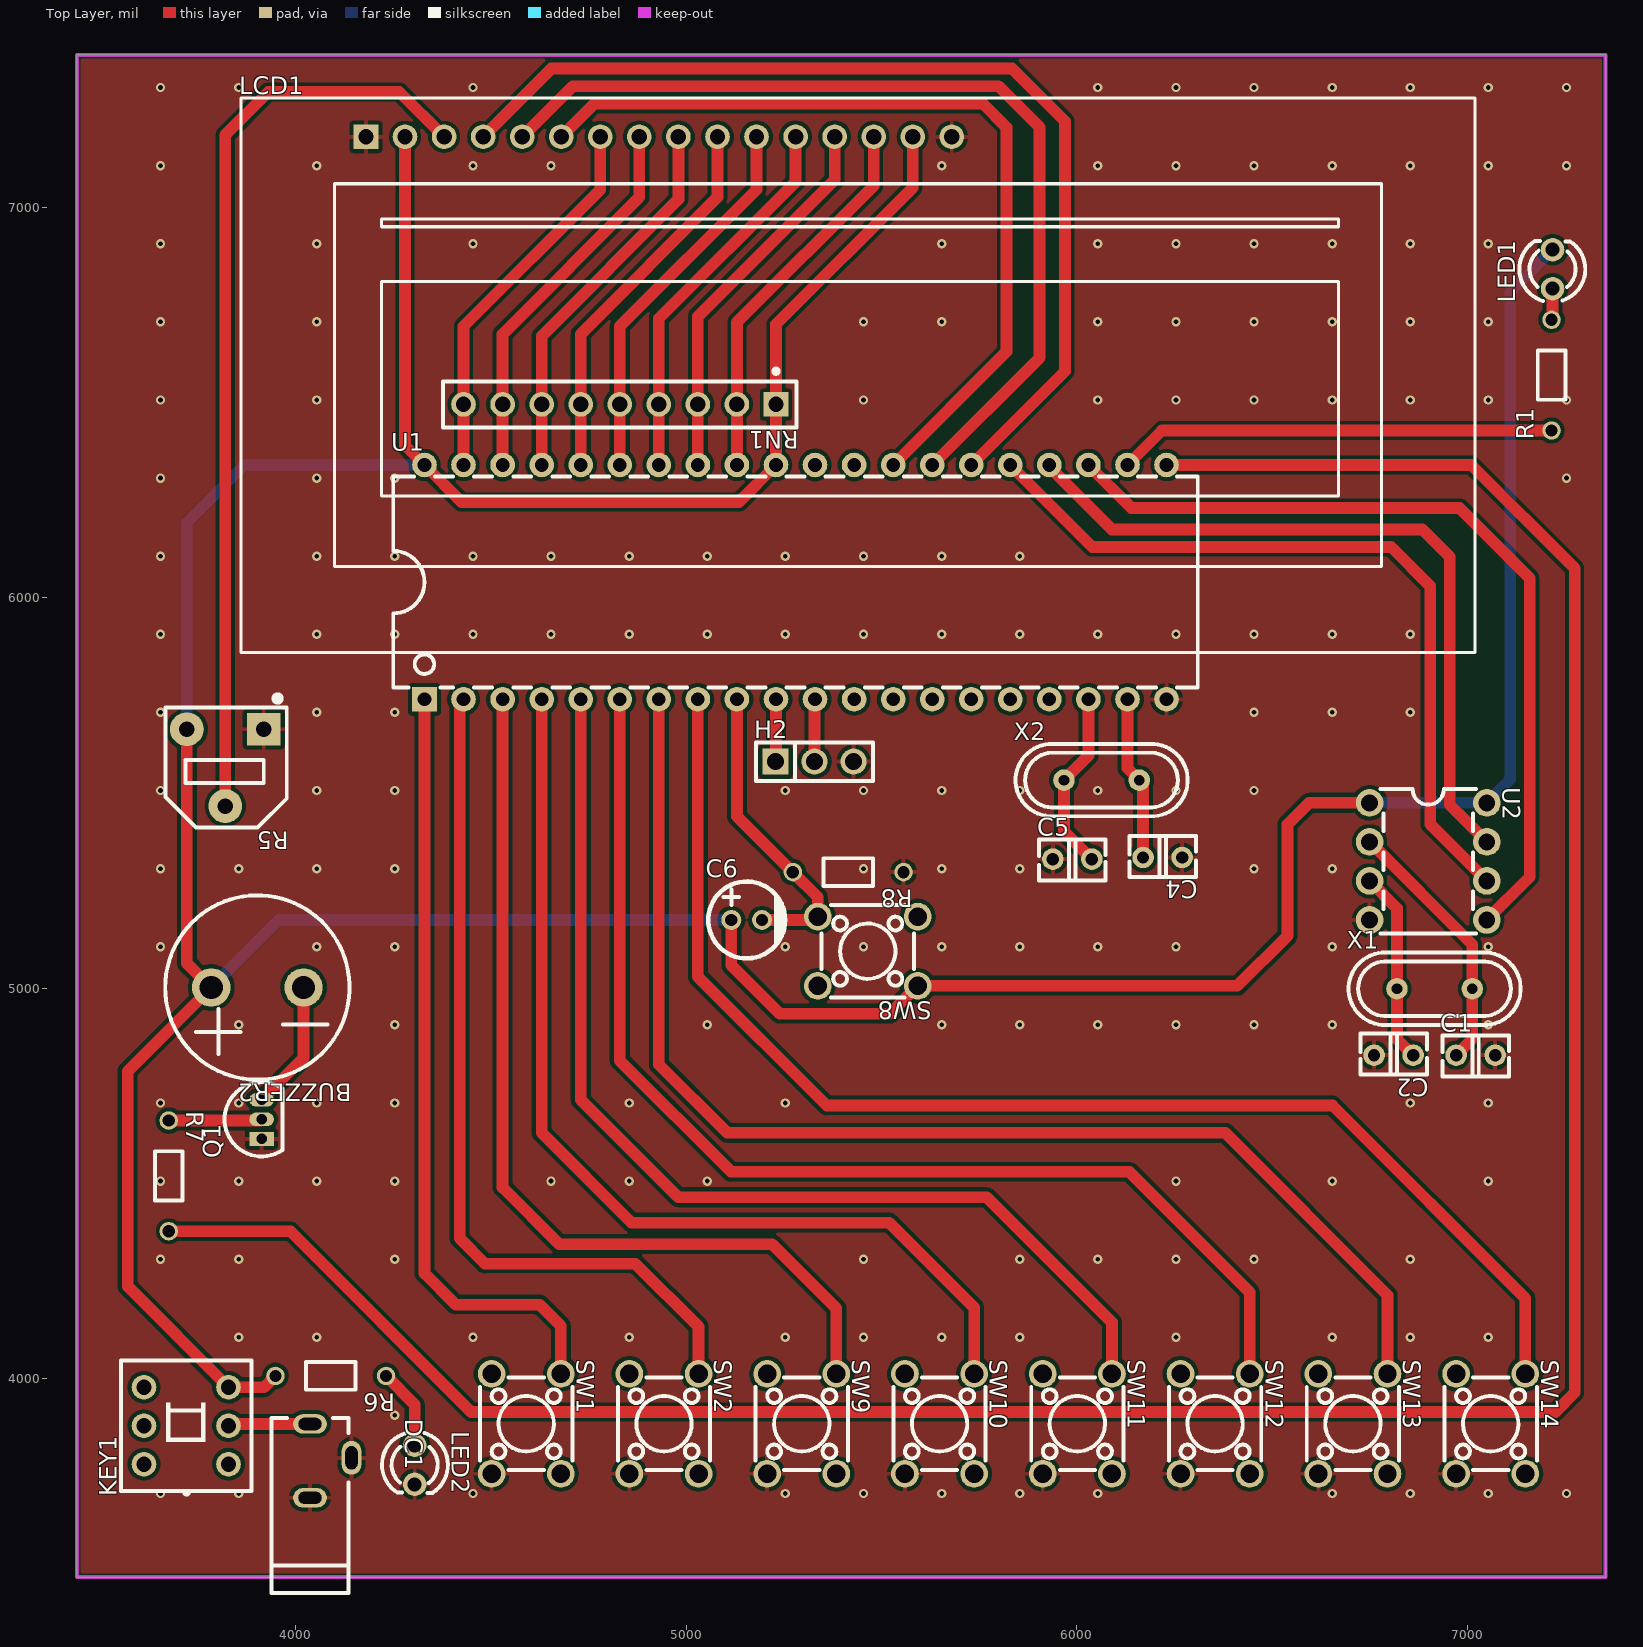
[diagram p0: Top Layer view]
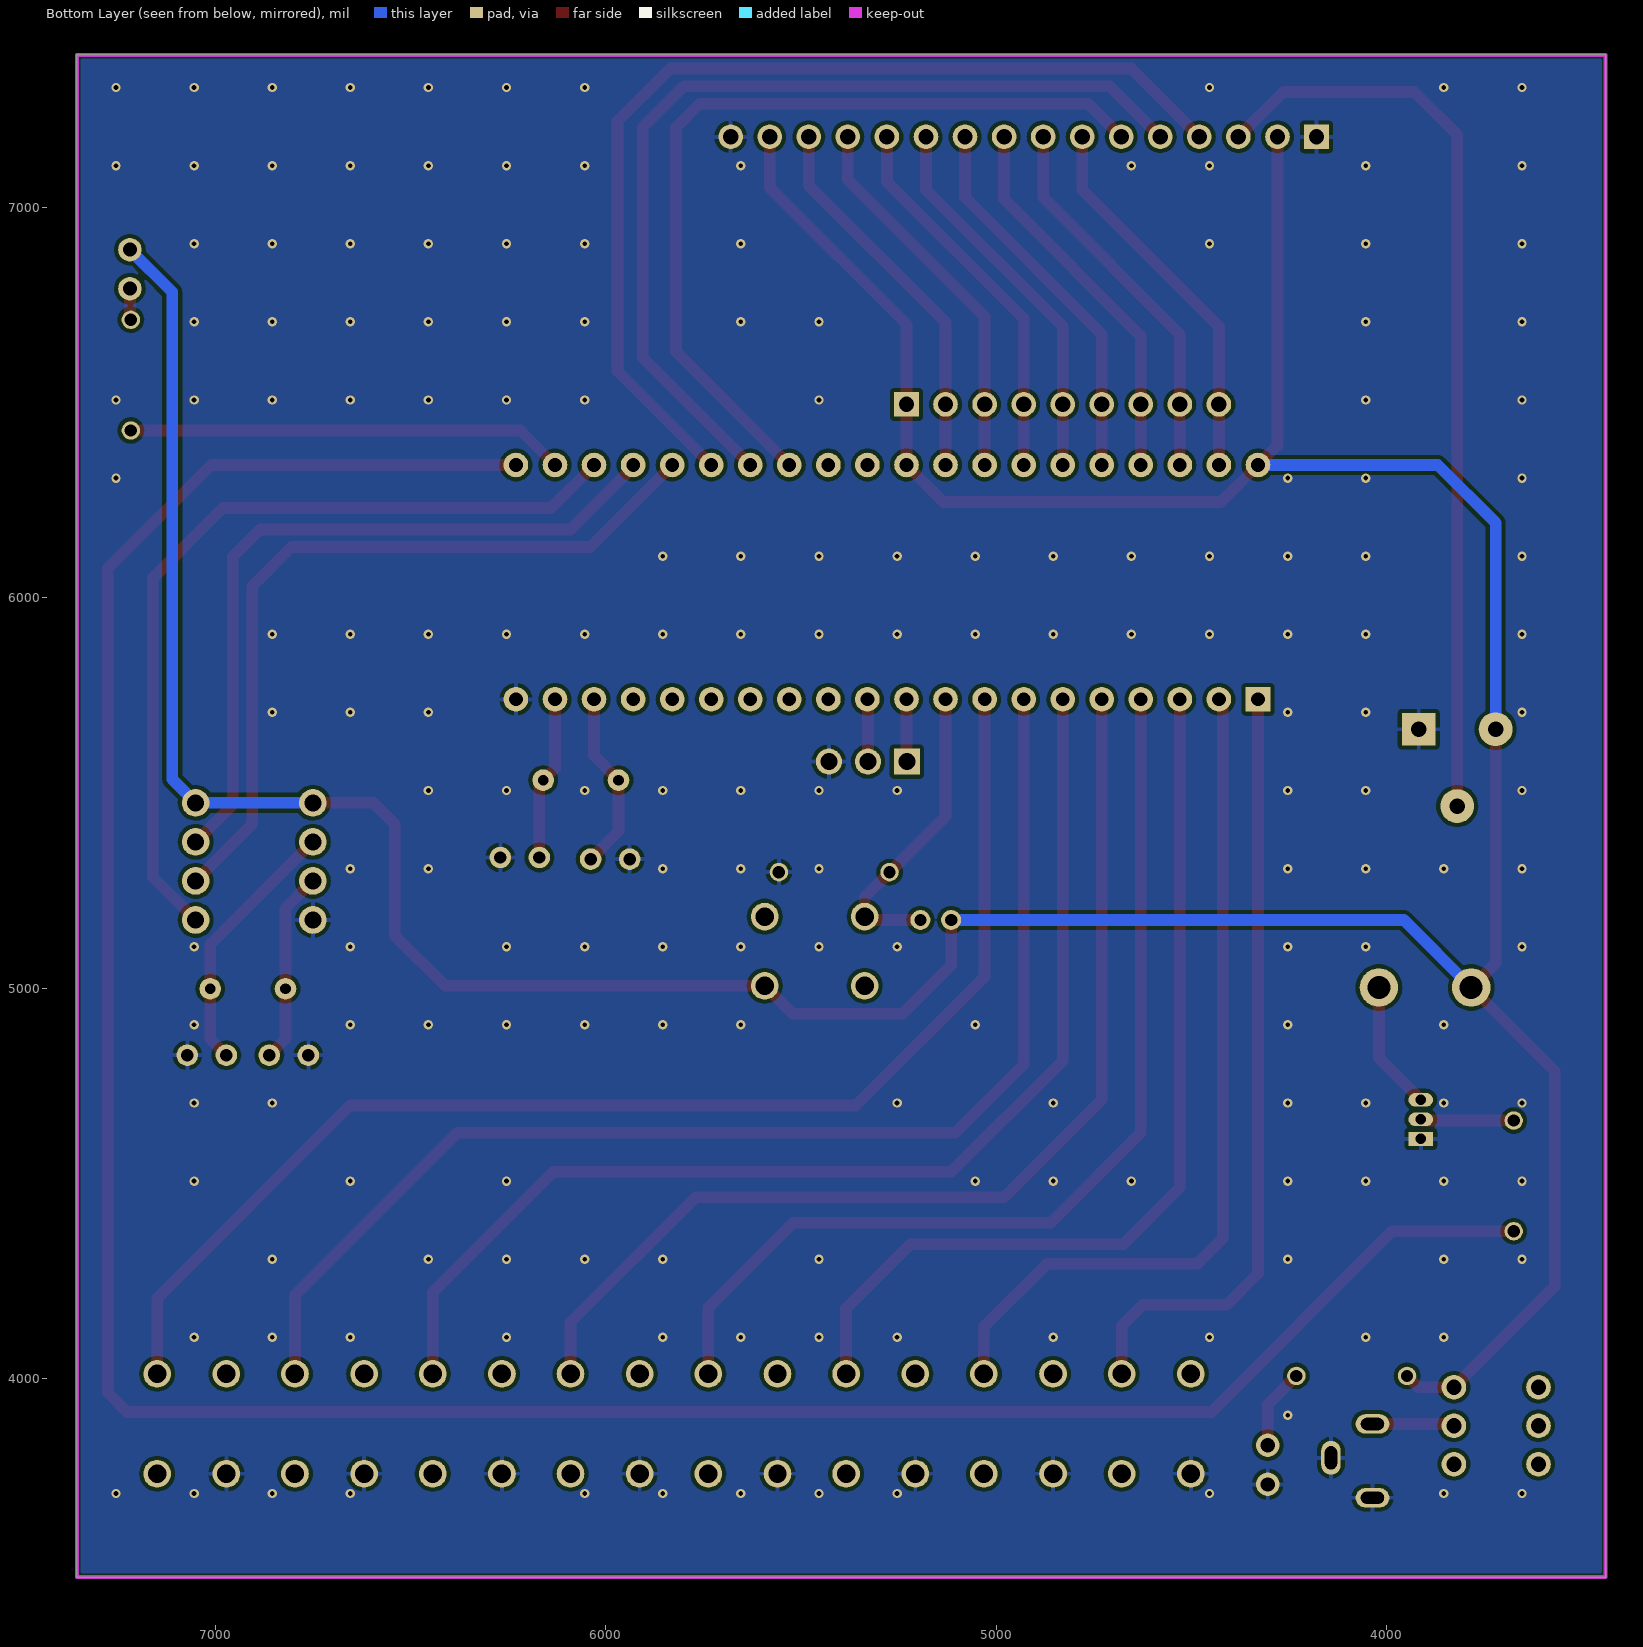
[diagram p1: Bottom Layer view, seen from below]
# Altium PCB MISC51000.pcbdoc
Units mil, origin at the board's own origin, x right, y up, seen from the top; angles counter-clockwise.
Board outline 3914.17 x 3897.64 mil, 2 copper layers (Top Layer, Bottom Layer), stack 62.206 mil thick; 32 components, 45 nets, 155 pads, 181 vias.

## Layer stack, top to bottom
Top Solder Mask Layer: solder mask 0.394, Dk 3.3
Top Layer: signal copper 1.379
Dielectric1: surface 59.449, FR4, Dk 4.5
Bottom Layer: signal copper 1.378
Bottom Solder Mask Layer: solder mask 0.394, Dk 3.3

## Board outline
3440,7390 3440,3492.36 7354.17,3492.36 7354.17,7390

## Design rules (kind name [scope] priority, off if disabled: settings)
BoardOutlineClearance copperThickness2oz_1 [All] p2 off: genericclearance=7.99 ignorepadtopadclearanceinfootprint=FALSE except(0: Arc-SplitContinuation Track-SplitContinuation SMDPad-SplitContinuation THPad-SplitContinuation Via-SplitContinuation Fill-SplitContinuation Region-SplitContinuation Poly-SplitContinuation Text-SplitContinuation Hole-SplitContinuation; 5.98: Arc-CutoutEdge SMDPad-CutoutEdge THPad-CutoutEdge Via-CutoutEdge Fill-CutoutEdge Region-CutoutEdge Text-CutoutEdge; 6.93: Hole-OutlineEdge Hole-CutoutEdge; 10: Poly-OutlineEdge Poly-CutoutEdge; 11.81: Arc-OutlineEdge Track-OutlineEdge SMDPad-OutlineEdge THPad-OutlineEdge Via-OutlineEdge Fill-OutlineEdge Region-OutlineEdge Text-OutlineEdge Track-CutoutEdge)
BoardOutlineClearance copperThickness1oz_1 [All] p4: genericclearance=4.02 ignorepadtopadclearanceinfootprint=FALSE except(0: Arc-SplitContinuation Track-SplitContinuation SMDPad-SplitContinuation THPad-SplitContinuation Via-SplitContinuation Fill-SplitContinuation Region-SplitContinuation Poly-SplitContinuation Text-SplitContinuation Hole-SplitContinuation; 6: SMDPad-CutoutEdge THPad-CutoutEdge Via-CutoutEdge Fill-CutoutEdge Region-CutoutEdge Text-CutoutEdge; 6.93: Hole-OutlineEdge Hole-CutoutEdge; 10: Poly-OutlineEdge Poly-CutoutEdge; 11.8: Arc-OutlineEdge Track-OutlineEdge SMDPad-OutlineEdge THPad-OutlineEdge Via-OutlineEdge Fill-OutlineEdge Region-OutlineEdge Text-OutlineEdge; 11.81: Arc-CutoutEdge Track-CutoutEdge)
Clearance copperThickness2oz [All] p1 off: gap=7.99 ignorepadtopadclearanceinfootprint=FALSE except(5.98: SMDPad-Track SMDPad-SMDPad THPad-Track SMDPad-THPad THPad-THPad Track-Via SMDPad-Via THPad-Via Via-Via Fill-Track Region-Track Fill-SMDPad Region-SMDPad Fill-THPad Region-THPad Fill-Via Region-Via Fill-Fill Fill-Region Region-Region Arc-Track Arc-SMDPad Arc-THPad Arc-Via Fill-Arc Region-Arc Arc-Arc Text-Track SMDPad-Text Text-THPad Text-Via Fill-Text Region-Text Arc-Text Text-Text; 6.93: Hole-Track Hole-SMDPad Hole-THPad Hole-Via Fill-Hole Region-Hole Hole-Arc Hole-Text; 10: Poly-Track Poly-SMDPad Poly-THPad Poly-Via Poly-Fill Poly-Region Poly-Poly Poly-Arc Poly-Text Poly-Hole)
Clearance copperThickness1oz [All] p3: gap=4.02 ignorepadtopadclearanceinfootprint=FALSE except(5.98: SMDPad-Track SMDPad-SMDPad THPad-Track SMDPad-THPad THPad-THPad Track-Via SMDPad-Via THPad-Via Via-Via Fill-Track Region-Track Fill-SMDPad Region-SMDPad Fill-THPad Region-THPad Fill-Via Region-Via Fill-Fill Fill-Region Region-Region; 6: Arc-Track Arc-SMDPad Arc-THPad Arc-Via Fill-Arc Region-Arc Arc-Arc Text-Track SMDPad-Text Text-THPad Text-Via Fill-Text Region-Text Arc-Text Text-Text; 6.93: Hole-Track Hole-SMDPad Hole-THPad Hole-Via Fill-Hole Region-Hole Hole-Arc Hole-Text; 10: Poly-Track Poly-SMDPad Poly-THPad Poly-Via Poly-Fill Poly-Region Poly-Poly Poly-Arc Poly-Text Poly-Hole)
Creepage creepage [All] p1: checkdistance=0 ignoreinternallayers=TRUE applytopolygonpour=TRUE
DiffPairsRouting differentialPair [All] p1: maxlimit=6 minlimit=6 mostfreqgap=6 toplayer_minwidth=5 toplayer_prefwidth=10 toplayer_maxwidth=100 toplayer_mingap=6 toplayer_prefgap=6 toplayer_maxgap=6 bottomlayer_minwidth=5 bottomlayer_prefwidth=10 bottomlayer_maxwidth=100 bottomlayer_mingap=6 bottomlayer_prefgap=6 bottomlayer_maxgap=6 maxuncoupledlength=10
HoleToHoleClearance otherClearance [All] p1: gap=11.81 allowstackedmicrovias=TRUE
Length netLength [All] p1: minlimit=0 maxlimit=0
MatchedLengths netLengthTolerance [All] p1: tolerance=1000
PasteMaskExpansion pasteMaskExpansion [All] p1: expansion=0
PlaneConnect innerPlane [All] p1: planeconnectstyle=Relief reliefexpansion=20 reliefentries=4 reliefconductorwidth=10 reliefairgap=10
PolygonConnect copperRegion [(InNet('GND'))] p1: connectstyle=Relief reliefconductorwidth=10 reliefentries=4 polygonreliefangle="90 Angle" airgapwidth=10 via.connectstyle=Relief via.reliefconductorwidth=10 via.reliefentries=4 via.polygonreliefangle="90 Angle" via.airgapwidth=10
RoutingVias viaSize [All] p1: holewidth=12.01 width=24.02 viastyle="Through Hole" minholewidth=11.81 minwidth=19.68 maxholewidth=248.03 maxwidth=393.7
SolderMaskExpansion solderMaskExpansion [IsVia] p1: expansion=-1000 istentingtop=TRUE
SolderMaskExpansion solderMaskExpansion [All] p2: expansion=2 istentingtop=FALSE
Width copperThickness2oz_2 [All] p1 off: maxlimit=100 minlimit=8 preferedwidth=10
Width copperThickness1oz_2 [All] p2: maxlimit=100 minlimit=5 preferedwidth=10

## Components (designator, comment, footprint, x,y, rotation, side; value= is the part's Value field where it differs from the comment)
BUZZER2 "buzzer" BUZ-TH_BD12.0-P6.00-D0.9-RD 3902.2,5002.04 r180 top
C1 "1nF" CAP-TH_L3.8-W2.5-P2.54-D0.50 7021.44,4828.83 r0 top
C2 "1nF" CAP-TH_L3.8-W2.5-P2.54-D0.50 6811.44,4828.83 r180 top
C4 "22pF" CAP-TH_L3.8-W2.5-P2.54-D0.50 6220,5335 r180 top
C5 "22pF" CAP-TH_L3.8-W2.5-P2.54-D0.50 5988.8,5330.73 r0 top
C6 "10uF" CAP-TH_BD5.0-P2.00-D0.8-FD-10UF50VC110GL 5155,5175 r0 top
DC1 "DC-002" DC-IN-TH_DC-3510 4090,3790 r270 top
H2 "" HDR-TH_3P-P2.54-V-M 5328.8,5580.46 r0 top
KEY1 "Non-latching switch 8.5×8.5 silent" SW-TH_6P-L8.5-W8.5-P2.54 3720,3880 r90 top
LCD1 "HS1602A" LCD1602 5440,6570 r0 top
LED1 "" LED_TH-3mm 7218.4,6841.27 r90 top
LED2 "" LED_TH-3mm 4305,3780 r270 top
Q1 "" S8050_TO_92 3913.08,4664.57 r90 top
R1 "100" Res_1/8W 7218.4,6570.02 r90 top
R5 "10kΩ" RES-ADJ-SMD_RM065-V1 3820,5565 r180 top
R6 "1kΩ" Res_1/8W 4090,4010 r180 top
R7 "10kΩ" Res_1/8W 3672.75,4519.71 r270 top
R8 "10kΩ" Res_1/8W 5415,5300 r180 top
RN1 "-" RES-ARRAY-TH_9P-P2.54-D1.0 4830,6495 r180 top
SW1 "" SW-TH_4P-L6.0-W6.0-P4.50-LS6.5 4590.5,3885 r270 top
SW2 "" SW-TH_4P-L6.0-W6.0-P4.50-LS6.5 4943.28,3885 r270 top
SW8 "" SW-TH_4P-L6.0-W6.0-P4.50-LS6.5 5465,5095 r180 top
SW9 "" SW-TH_4P-L6.0-W6.0-P4.50-LS6.5 5296.07,3885 r270 top
SW10 "" SW-TH_4P-L6.0-W6.0-P4.50-LS6.5 5648.85,3885 r270 top
SW11 "" SW-TH_4P-L6.0-W6.0-P4.50-LS6.5 6001.64,3885 r270 top
SW12 "" SW-TH_4P-L6.0-W6.0-P4.50-LS6.5 6354.43,3885 r270 top
SW13 "" SW-TH_4P-L6.0-W6.0-P4.50-LS6.5 6707.21,3885 r270 top
SW14 "" SW-TH_4P-L6.0-W6.0-P4.50-LS6.5 7060,3885 r270 top
U1 "STC89C52RC-40I-PDIP40" DIP-40_L52.0-W13.7-P2.54-LS15.2-BL 5280,6040 r0 top
U2 "DS1302N(XBLW)" PDIP-8_L9.3-W6.4-P2.54-LS7.6-BL 6900,5325 r270 top
X1 "11.0592MHz" OSC-TH_L11.1-W4.7-P4.88 6916.44,4998.83 r0 top
X2 "11.0592MHz" OSC-TH_L11.1-W4.7-P4.88 6063.8,5533.02 r0 top

## Footprints (in the part's own frame and the unit in brackets; to place one, negate y for a bottom-side part, rotate by r counter-clockwise, add the part's x,y. Pads: shape width x height; smd on the part's side, far side on the other; paste and mask are expansions set on the pad)
BUZ-TH_BD12.0-P6.00-D0.9-RD [mm]
  round 2.5 hole 1.5 paste+0 mask+0.05: 1(-3,0) 2(3,0)
  silkscreen extent -5.99,-5.99 5.99,5.99
CAP-TH_BD5.0-P2.00-D0.8-FD-10UF50VC110GL [mm]
  round 1.3 hole 0.8: 1(-1,0) 2(1,0)
  silkscreen extent -2.5,-2.5 2.5,2.5
CAP-TH_L3.8-W2.5-P2.54-D0.50 [mm]
  round 1.4 hole 0.8 paste+0 mask+0.05: 1(-1.27,0) 2(1.27,0)
  silkscreen extent -2.16,-1.4 2.16,1.27
DC-IN-TH_DC-3510 [mm]
  oval 1.27x2.2 hole 0.8 slot 1.5 at 90 deg: 1(-2.4,-1.35) 2(2.4,-1.35)
  oval 2.2x1.27 hole 0.8 slot 1.5 at 0 deg: 3(-0.2,1.35)
  silkscreen extent -2.8,-3.85 8.6,1.15
DIP-40_L52.0-W13.7-P2.54-LS15.2-BL [mil]
  rect 63x63 hole 35: 1(-950,-300)
  round 63 hole 35: 2(-850,-300) 3(-750,-300) 4(-650,-300) 5(-550,-300) 6(-450,-300) 7(-350,-300) 8(-250,-300) 9(-150,-300) 10(-50,-300) 11(50,-300) 12(150,-300) 13(250,-300) 14(350,-300) 15(450,-300) 16(550,-300) 17(650,-300) 18(750,-300) 19(850,-300) 20(950,-300) 21(950,300) 22(850,300) 23(750,300) 24(650,300) 25(550,300) 26(450,300) 27(350,300) 28(250,300) 29(150,300) 30(50,300) 31(-50,300) 32(-150,300) 33(-250,300) 34(-350,300) 35(-450,300) 36(-550,300) 37(-650,300) 38(-750,300) 39(-850,300) 40(-950,300)
  silkscreen extent -1030,-270 1030,270
HDR-TH_3P-P2.54-V-M [mm]
  rect 1.7x1.7 hole 1.1: 1(-2.54,0)
  round 1.7 hole 1.1: 2(0,0) 3(2.54,0)
  silkscreen extent -3.81,-1.25 3.81,1.25
LCD1602 [mm]
  rect 1.6x1.6 hole 1: 1(-32,15.5)
  round 1.6 hole 1: 2(-29.46,15.5) 3(-26.92,15.5) 4(-24.38,15.5) 5(-21.84,15.5) 6(-19.3,15.5) 7(-16.76,15.5) 8(-14.22,15.5) 9(-11.68,15.5) 10(-9.14,15.5) 11(-6.6,15.5) 12(-4.06,15.5) 13(-1.52,15.5) 14(1.02,15.5) 15(3.56,15.5) 16(6.1,15.5)
  silkscreen extent -40.13,-18.03 40.13,18.03
LED_TH-3mm [mil]
  round 60 hole 36 paste+0 mask+2: 1(-50,0) 2(50,0)
  silkscreen extent -81,-84 72,85
OSC-TH_L11.1-W4.7-P4.88 [mm]
  round 1.4 hole 0.7: 1(-2.45,0) 2(2.45,0)
  silkscreen extent -5.59,-2.35 5.6,2.35
PDIP-8_L9.3-W6.4-P2.54-LS7.6-BL [mm]
  round 1.8 hole 1.1: 1(-3.81,-3.81) 2(-1.27,-3.81) 3(1.27,-3.81) 4(3.81,-3.81) 5(3.81,3.81) 6(1.27,3.81) 7(-1.27,3.81) 8(-3.81,3.81)
  silkscreen extent -4.7,-3.11 4.7,3.11
RES-ADJ-SMD_RM065-V1 [mm]
  rect 2.2x2.1 hole 1 paste+0 mask+0.05: 1(-2.5,-2.5)
  round 2.2 hole 1 paste+0 mask+0.05: 2(0,2.5) 3(2.5,-2.5)
  silkscreen extent -4,-4.7 3.9,3.9
RES-ARRAY-TH_9P-P2.54-D1.0 [mm]
  rect 1.6x1.6 hole 1: 1(-10.16,0)
  round 1.6 hole 1: 2(-7.62,0) 3(-5.08,0) 4(-2.54,0) 5(0,0) 6(2.54,0) 7(5.08,0) 8(7.62,0) 9(10.16,0)
  silkscreen extent -11.5,-2.31 11.5,1.5
Res_1/8W [mil]
  round 47.2 hole 31.5 paste+0 mask+2: 1(-141.7,2.48) 2(141.7,2.48)
  silkscreen extent -63,-33 63,38
S8050_TO_92 [mil]
  rect 35.4x63 hole 27.6 paste+0 mask+2: 1(-50,0)
  oval 35.4x63 hole 27.6 paste+0 mask+2: 2(0,0) 3(50,0)
  silkscreen extent -95,-53 95,95
SW-TH_4P-L6.0-W6.0-P4.50-LS6.5 [mm]
  round 1.8 hole 1.2: 1(-3.25,2.25) 2(3.25,2.25) 3(-3.25,-2.25) 4(3.25,-2.25)
  silkscreen extent -3,-3 3,3
SW-TH_6P-L8.5-W8.5-P2.54 [mm]
  round 1.6 hole 1: 1(-2.5,-2.75) 2(0,-2.75) 3(2.5,-2.75) 4(-2.5,2.75) 5(0,2.75) 6(2.5,2.75)
  silkscreen extent -4.47,-4.25 4.25,4.25

## Via types
v1: diameter 24.02, hole 12, Top Layer to Bottom Layer, 181 vias

## Nets (pads, with @x,y where several pads share a name; then routed paths per layer and width w, separated by ;. In a path a pad name is that pad's centre, name@x,y a point inside that pad or via, vN(x,y) a via of type N, cw(c..) or ccw(c..) an arc to the next point about the centre after c; other vN are vias at no path point)
$1N95: Q1.2 R7.1 | length 239.2
  Top Layer w30: R7.1 3909.93,4661.41 Q1.2
$1N111: LED2.1 R6.1 | length 207.9
  Top Layer w30: R6.1 4305,3934.22 LED2.1
$1N113: DC1.1 KEY1.2 | length 210.4
  Top Layer w30: KEY1.2 3832.76,3884.49 DC1.1
$1N115: LCD1.3 R5.2 | length 2371.7
  Top Layer w30: R5.2 3820,7185 3930,7295 4265.4,7295 LCD1.3
$1N167: BUZZER2.1 Q1.3 | length 331.9
  Top Layer w30: Q1.3 4020.31,4821.8 BUZZER2.1
$1N169: LED1.1 R1.2 | length 80.6
  Top Layer w30: R1.2 7218.4,6714.2 LED1.1
$1N174: C1.1 U2.2 X1.2 | length 672.2
  Top Layer w30: U2.2 7012.89,5112.11 X1.2 7012.89,4870.28 C1.1
$1N175: C2.1 U2.3 X1.1 | length 492.3
  Top Layer w30: U2.3 6819.99,5205.01 X1.1 6819.99,4870.28 C2.1
GND: C1.2 C2.2 C4.1 C5.1 DC1.2 DC1.3 H2.3 LCD1.1 LCD1.16 LED2.2 Q1.1 R5.1 R8.1 SW1.4 SW2.4 SW9.4 SW10.4 SW11.4 SW12.4 SW13.4 SW14.4 U1.20 U2.4
  other v1: 3654.1,3706.46 3854.1,3706.46 4454.1,3706.46 5254.1,3706.46 5454.1,3706.46 5654.1,3706.46 5854.1,3706.46 6054.1,3706.46 6654.1,3706.46 6854.1,3706.46 7054.1,3706.46 7254.1,3706.46 4254.1,3906.46 3854.1,4106.46 4054.1,4106.46 4454.1,4106.46 4854.1,4106.46 5254.1,4106.46 5454.1,4106.46 5654.1,4106.46 5854.1,4106.46 6254.1,4106.46 6654.1,4106.46 6854.1,4106.46 7054.1,4106.46 3654.1,4306.46 3854.1,4306.46 4254.1,4306.46 5454.1,4306.46 5854.1,4306.46 6054.1,4306.46 6254.1,4306.46 6454.1,4306.46 6854.1,4306.46 3654.1,4506.46 3854.1,4506.46 4054.1,4506.46 4254.1,4506.46 4654.1,4506.46 4854.1,4506.46 5054.1,4506.46 6254.1,4506.46 6654.1,4506.46 7054.1,4506.46 3654.1,4706.46 3854.1,4706.46 4054.1,4706.46 4254.1,4706.46 4854.1,4706.46 5254.1,4706.46 6854.1,4706.46 7054.1,4706.46 3854.1,4906.46 4254.1,4906.46 5054.1,4906.46 5654.1,4906.46 5854.1,4906.46 6054.1,4906.46 6254.1,4906.46 6454.1,4906.46 6654.1,4906.46 7054.1,4906.46 3654.1,5106.46 4054.1,5106.46 4254.1,5106.46 5254.1,5106.46 5454.1,5106.46 5654.1,5106.46 5854.1,5106.46 6054.1,5106.46 6254.1,5106.46 6654.1,5106.46 7054.1,5106.46 3654.1,5306.46 3854.1,5306.46 4054.1,5306.46 4254.1,5306.46 5454.1,5306.46 5654.1,5306.46 5854.1,5306.46 6454.1,5306.46 6654.1,5306.46 3654.1,5506.46 4054.1,5506.46 4254.1,5506.46 5254.1,5506.46 5454.1,5506.46 5654.1,5506.46 5854.1,5506.46 6054.1,5506.46 6254.1,5506.46 6454.1,5506.46 3654.1,5706.46 4054.1,5706.46 4254.1,5706.46 6454.1,5706.46 6654.1,5706.46 6854.1,5706.46 3654.1,5906.46 4054.1,5906.46 4254.1,5906.46 4454.1,5906.46 4654.1,5906.46 4854.1,5906.46 5054.1,5906.46 5254.1,5906.46 5454.1,5906.46 5654.1,5906.46 5854.1,5906.46 6054.1,5906.46 6254.1,5906.46 6454.1,5906.46 6654.1,5906.46 6854.1,5906.46 3654.1,6106.46 4054.1,6106.46 4254.1,6106.46 4454.1,6106.46 4654.1,6106.46 4854.1,6106.46 5054.1,6106.46 5254.1,6106.46 5454.1,6106.46 5654.1,6106.46 5854.1,6106.46 3654.1,6306.46 4054.1,6306.46 4254.1,6306.46 7254.1,6306.46 3654.1,6506.46 4054.1,6506.46 5454.1,6506.46 6054.1,6506.46 6254.1,6506.46 6454.1,6506.46 6654.1,6506.46 6854.1,6506.46 7054.1,6506.46 7254.1,6506.46 3654.1,6706.46 4054.1,6706.46 5454.1,6706.46 5654.1,6706.46 6054.1,6706.46 6254.1,6706.46 6454.1,6706.46 6654.1,6706.46 6854.1,6706.46 7054.1,6706.46 3654.1,6906.46 4054.1,6906.46 4454.1,6906.46 5654.1,6906.46 6054.1,6906.46 6254.1,6906.46 6454.1,6906.46 6654.1,6906.46 6854.1,6906.46 7054.1,6906.46 3654.1,7106.46 4054.1,7106.46 4454.1,7106.46 4654.1,7106.46 5654.1,7106.46 6054.1,7106.46 6254.1,7106.46 6454.1,7106.46 6654.1,7106.46 6854.1,7106.46 7054.1,7106.46 7254.1,7106.46 3654.1,7306.46 3854.1,7306.46 4454.1,7306.46 6054.1,7306.46 6254.1,7306.46 6454.1,7306.46 6654.1,7306.46 6854.1,7306.46 7054.1,7306.46 7254.1,7306.46
P00: LCD1.7 RN1.9 U1.39 | length 985.3
  Top Layer w30: U1.39 RN1.9 4430,6695 4780.16,7045.16 LCD1.7
P01: LCD1.8 RN1.8 U1.38 | length 985.3
  Top Layer w30: U1.38 RN1.8 4530,6675 4880.16,7025.16 LCD1.8
P02: LCD1.9 RN1.7 U1.37 | length 985.3
  Top Layer w30: U1.37 RN1.7 4630,6670 4980.16,7020.16 LCD1.9
P03: LCD1.10 RN1.6 U1.36 | length 985.3
  Top Layer w30: U1.36 RN1.6 4730,6675 5080.16,7025.16 LCD1.10
P04: LCD1.11 RN1.5 U1.35 | length 985.3
  Top Layer w30: U1.35 RN1.5 4830,6695 5180.16,7045.16 LCD1.11
P05: LCD1.12 RN1.4 U1.34 | length 985.3
  Top Layer w30: U1.34 RN1.4 4930,6715 5280.16,7065.16 LCD1.12
P06: LCD1.13 RN1.3 U1.33 | length 985.3
  Top Layer w30: U1.33 RN1.3 5030,6720 5380.16,7070.16 LCD1.13
P07: LCD1.14 RN1.2 U1.32 | length 985.3
  Top Layer w30: U1.32 RN1.2 5130,6705 5480.16,7055.16 LCD1.14
P10: SW1.1 U1.1 | length 1997.6
  Top Layer w30: U1.1 4330,4270 4410,4190 4625,4190 4679.08,4135.92 SW1.1
P11: SW2.1 U1.2 | length 2210.2
  Top Layer w30: U1.2 4420,5730 4420,4360 4485,4295 4870,4295 5031.86,4133.14 SW2.1
P12: SW9.1 U1.3 | length 2400.3
  Top Layer w30: U1.3 4530,4490 4675,4345 5220,4345 5384.65,4180.35 SW9.1@5384.65,4012.95
P13: SW10.1 U1.4 | length 2572.4
  Top Layer w30: U1.4 4630,4630 4860,4400 5520,4400 5737.44,4182.56 SW10.1
P14: SW11.1 U1.5 | length 2753.2
  Top Layer w30: U1.5 4730,4715 4980,4465 5770,4465 6090.22,4144.78 SW11.1
P15: SW12.1 U1.6 | length 2992.7
  Top Layer w30: U1.6 4830,4815 5115,4530 6135,4530 6443.01,4221.99 SW12.1
P16: SW13.1 U1.7 | length 3246.8
  Top Layer w30: U1.7 4930,4805 5105,4630 6380,4630 6795.79,4214.21 SW13.1
P17: SW14.1 U1.8 | length 3363.2
  Top Layer w30: U1.8 5030,5030 5360,4700 6655,4700 7148.58,4206.42 SW14.1
P20: R7.2 U1.21 | length 7077
  Top Layer w30: R7.2 3986.99,4378.01 4450,3915 7225,3915 7275,3965 7275,6075 7010,6340 U1.21
P21: R1.1 U1.22 | length 1122.5
  Top Layer w30: U1.22 6218.32,6428.32 R1.1
P22: U1.23 U2.5 | length 2170.7
  Top Layer w30: U1.23 6140,6230 6980,6230 7160,6050 7160,5285 U2.5
P23: U1.24 U2.7 | length 1894.6
  Top Layer w30: U1.24 5930,6335 6090,6175 6885,6175 6955,6105 6955,5470 U2.7
P24: U1.25 U2.6 | length 2018.5
  Top Layer w30: U1.25 6040,6130 6805,6130 6905,6030 6905,5420 U2.6
P25: LCD1.4 U1.26 | length 2597.6
  Top Layer w30: LCD1.4 4654.92,7355 5835,7355 5970,7220 5970,6580 U1.26
P26: LCD1.5 U1.27 | length 2401
  Top Layer w30: LCD1.5 4709.92,7310 5800,7310 5905,7205 5905,6615 U1.27
P27: LCD1.6 U1.28 | length 2184.9
  Top Layer w30: LCD1.6 4764.92,7265 5760,7265 5820,7205 5820,6630 U1.28
P30: H2.1 U1.10 | length 160
  Top Layer w30: H2.1 5230,5581.65 U1.10
P31: H2.2 U1.11 | length 160
  Top Layer w30: H2.2 5328.8,5738.8 U1.11
P32: U1.12
P33: U1.13
P34: U1.14
P35: U1.15
P36: U1.16
P37: U1.17
RST: C6.2 R8.2 SW8.4 U1.9 | length 788.4
  Top Layer w30: U1.9 5130,5440.82 R8.2 5337.05,5233.77 SW8.4 5328.47,5175 C6.2
VCC: BUZZER2.2 C6.1 KEY1.3 LCD1.2 LCD1.15 LED1.2 R5.3 R6.2 RN1.1 SW8.1 U1.31 U1.40 U2.1 U2.8 | length 11442.9
  Top Layer w30: R5.3 3721.57,5064.55 BUZZER2.2 3570,4787.95 3570,4236.69 KEY1.3 3919.2,3978.43 R6.2 ; LCD1.2 4280.16,6389.84 U1.40 4425,6245 5135,6245 U1.31 RN1.1 5230,6700 5580.16,7050.16 LCD1.15 ; C6.1 5115.63,5059.37 5240,4935 5521.53,4935 SW8.1 6411.42,5006.42 6540,5135 6540,5420 6595,5475 U2.1
  Bottom Layer w30: R5.3 3721.57,6191.57 3870,6340 U1.40 ; BUZZER2.2 3957.05,5175 C6.1 ; U2.1 U2.8 7110,5535 7110,6782.87 LED1.2
X1: C5.2 U1.18 X2.1 | length 464.8
  Top Layer w30: U1.18 6030,5595.67 X2.1 5967.35,5402.18 C5.2
X2: C4.2 U1.19 X2.2 | length 421.6
  Top Layer w30: U1.19 6130,5563.28 X2.2 6170,5523.28 C4.2
pads on no net: KEY1.1 KEY1.4 KEY1.5 KEY1.6 SW1.2 SW1.3 SW2.2 SW2.3 SW8.2 SW8.3 SW9.2 SW9.3 SW10.2 SW10.3 SW11.2 SW11.3 SW12.2 SW12.3 SW13.2 SW13.3 SW14.2 SW14.3 U1.29 U1.30

## Polygon pours and split planes (outlines as drawn)
GND on Bottom Layer (solid, remove dead copper, pour order 2): 3000,7935 3000,3000 7820,3000 7820,7935
GND on Top Layer (solid, remove dead copper, pour order 0): 3170,7730 3170,3240 7705,3240 7705,7730

## Keep-outs
Board Outline Layer:
  the board outline again, w10